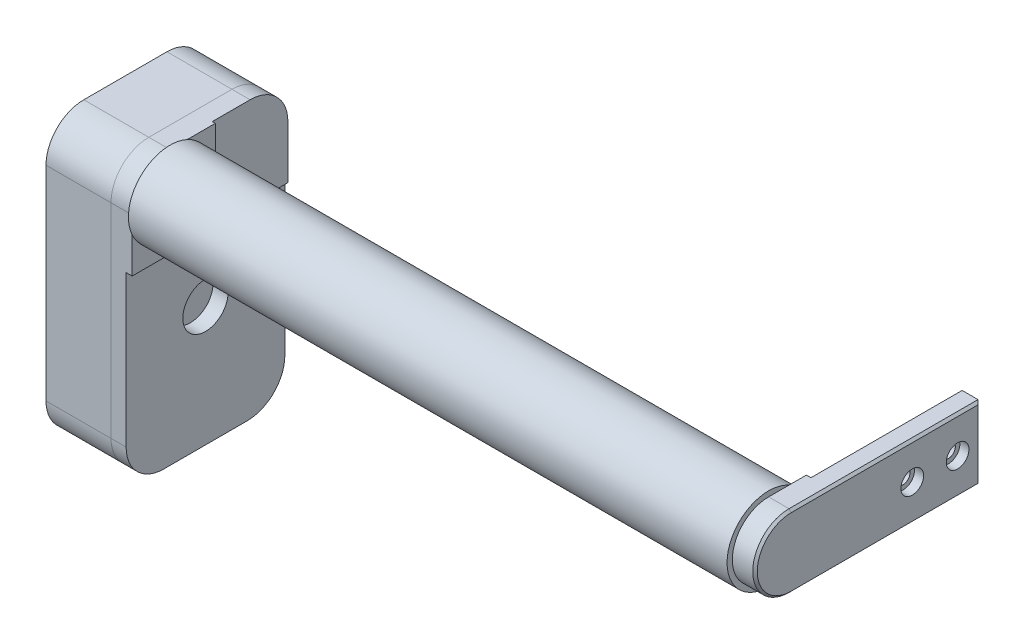
SolidWorks part; units mm, degrees
material "6061 合金"
ref_plane "前视基准面" through (0, 0, 0) normal (0, 0, 1) x (1, 0, 0)
ref_plane "上视基准面" through (0, 0, 0) normal (0, 1, 0) x (1, 0, 0)
ref_plane "右视基准面" through (0, 0, 0) normal (1, 0, 0) x (0, 0, -1)
sketch "草图1" plane through (0, 0, 0) normal (1, 0, 0) x (0, 0, -1)
  line L1 (-62.5, 24) -> (62.5, 24)
  line L2 (-62.5, 24) -> (-62.5, -24) construction
  line L3 (-62.5, -24) -> (62.5, -24)
  line L4 (62.5, 24) -> (62.5, -24)
  line L5 (-62.5, 24) -> (62.5, -24) construction
  line L6 (-62.5, -24) -> (62.5, 24) construction
  arc A0 (-62.5, 24) -> (-62.5, -24) centre (-62.5, 0) ccw
  point P0 (0, 0)
  dimension "D1" = 48
  dimension "D2" = 125
extrude "凸台-拉伸1" add sketch "草图1" along normal blind 15
sketch "草图2" plane through (0, 0, 0) normal (-1, 0, 0) x (0, 0, 1)
  circle A0 centre (62.5, 0) radius 27.5
  dimension "D1" = 55
extrude "凸台-拉伸2" add sketch "草图2" along normal blind 396
hole_wizard "打孔尺寸(%根据)内六角花形圆柱头螺钉1" positions "草图3" profile "草图4" counterbore size "M8" standard "GB" end condition through all
sketch "草图3" plane through (15, 0, 0) normal (1, 0, 0) x (0, 0, -1)
  line L0 (62.5, 0) -> (-4.2393, 0) construction
  line L1 (62.5, -24) -> (62.5, 24) construction
  point P0 (17.5, 0)
  point P2 (47.5, 0)
  dimension "D1" = 15
  dimension "D2" = 30
sketch "草图4" plane through (15, 0, -17.5) normal (0, 1, 0) x (0, 0, -1)
  line L0 (0, 0) -> (0, 411)
  line L1 (0, 411) -> (4.5, 411)
  line L3 (4.5, 411) -> (4.5, 6)
  line L4 (4.5, 6) -> (7.5, 6)
  line L5 (7.5, 6) -> (7.5, 0)
  line L7 (7.5, 0) -> (0, 0)
  line L11 (0, -6.35) -> (0, 107.95) construction
  dimension "通孔孔直径" = 9
  dimension "通孔孔深度" = 411
  dimension "柱形沉头孔直径" = 15
  dimension "柱形沉头孔深度" = 6
chamfer "倒角1" distance 1.5 angle 45 4 edges at (15, 0, -62.5) (15, -24, 0) (15, 0, 86.5) (15, 24, 0)
ref_plane "基准面1" through (-198, 0, 0) normal (-1, 0, 0) x (0, 0, 1)
sketch "草图5" plane through (0, 24, 0) normal (0, 1, 0) x (1, 0, 0)
  line L1 (0, 62.5) -> (3, 62.5)
  line L2 (0, 62.5) -> (0, -37.5)
  line L3 (0, -37.5) -> (3, -37.5)
  line L4 (3, 62.5) -> (3, -37.5)
  dimension "D1" = 100
  dimension "D2" = 3
extrude "切除-拉伸1" cut sketch "草图5" against normal through all
sketch "草图6" plane through (-396, 0, 0) normal (-1, 0, 0) x (0, 0, 1)
  circle A0 centre (62.5, 0) radius 8
  dimension "D1" = 16
extrude "凸台-拉伸3" add sketch "草图6" along normal blind 25
sketch "草图7" plane through (-396, 0, 0) normal (-1, 0, 0) x (0, 0, 1)
  line L1 (7.5, 25) -> (62.5, 25)
  line L2 (-17.5, 0) -> (-17.5, -135)
  line L3 (7.5, -160) -> (62.5, -160)
  line L4 (87.5, 0) -> (87.5, -135)
  arc A0 (62.5, 25) -> (87.5, 0) centre (62.5, 0) cw
  arc A1 (-17.5, -135) -> (7.5, -160) centre (7.5, -135) ccw
  arc A2 (62.5, -160) -> (87.5, -135) centre (62.5, -135) ccw
  arc A3 (7.5, 25) -> (-17.5, 0) centre (7.5, 0) ccw
  circle A4 centre (62.5, 0) radius 27.5 construction
  point P6 (87.5, 25)
  point P9 (-17.5, -160)
  point P14 (-17.5, 25)
  dimension "D3" = 25
  dimension "D1" = 105
  dimension "D2" = 185
extrude "凸台-拉伸4" add sketch "草图7" along normal blind 14
sketch "草图8" plane through (0, 0, -17.5) normal (0, 0, -1) x (-1, 0, 0)
  line L0 (396, 0) -> (396, -135) construction
  line L1 (396, -35) -> (400, -35)
  line L2 (396, -35) -> (396, -160)
  line L3 (396, -160) -> (400, -160)
  line L4 (400, -35) -> (400, -160)
  line L5 (410, -160) -> (396, -160) construction
  dimension "D1" = 4
  dimension "D2" = 125
extrude "切除-拉伸2" cut sketch "草图8" against normal through all
sketch "草图9" plane through (-400, 0, 0) normal (1, 0, 0) x (0, 0, -1)
  line L0 (-35, -160) -> (-35, -35) construction
  line L1 (-62.5, -160) -> (-7.5, -160) construction
  line L2 (-87.5, -35) -> (17.5, -35) construction
  circle A0 centre (-35, -80) radius 15
  dimension "D1" = 80
  dimension "D2" = 30
extrude "切除-拉伸3" cut sketch "草图9" against normal through all
sketch "草图10" plane through (0, 25, 0) normal (0, 1, 0) x (1, 0, 0)
  line L0 (-396, -51.0436) -> (-396, -7.5) construction
  line L1 (-396, -32.5) -> (-398, -32.5)
  line L2 (-396, -32.5) -> (-396, 17.5)
  line L3 (-396, 17.5) -> (-398, 17.5)
  line L4 (-398, -32.5) -> (-398, 17.5)
  line L5 (-410, 17.5) -> (-396, 17.5) construction
  dimension "D1" = 50
  dimension "D2" = 2
extrude "切除-拉伸4" cut sketch "草图10" against normal through all
sketch "草图11" plane through (-410, 0, 0) normal (-1, 0, 0) x (0, 0, 1)
  line L4 (62.5, 25) -> (7.5, 25)
  line L5 (-17.5, 0) -> (-17.5, -135)
  line L6 (7.5, -160) -> (62.5, -160)
  line L7 (87.5, -135) -> (87.5, 0)
  line L8 (62.5, 25) -> (7.5, 25)
  line L9 (-17.5, 0) -> (-17.5, -135)
  line L10 (7.5, -160) -> (62.5, -160)
  line L11 (87.5, -135) -> (87.5, 0)
  arc A4 (87.5, 0) -> (62.5, 25) centre (62.5, 0) ccw
  arc A5 (7.5, 25) -> (-17.5, 0) centre (7.5, 0) ccw
  arc A6 (-17.5, -135) -> (7.5, -160) centre (7.5, -135) ccw
  arc A7 (62.5, -160) -> (87.5, -135) centre (62.5, -135) ccw
  arc A8 (87.5, 0) -> (62.5, 25) centre (62.5, 0) ccw
  arc A9 (7.5, 25) -> (-17.5, 0) centre (7.5, 0) ccw
  arc A10 (-17.5, -135) -> (7.5, -160) centre (7.5, -135) ccw
  arc A11 (62.5, -160) -> (87.5, -135) centre (62.5, -135) ccw
  dimension "D1" = 0
extrude "凸台-拉伸5" add sketch "草图11" along normal blind 43 separate body
